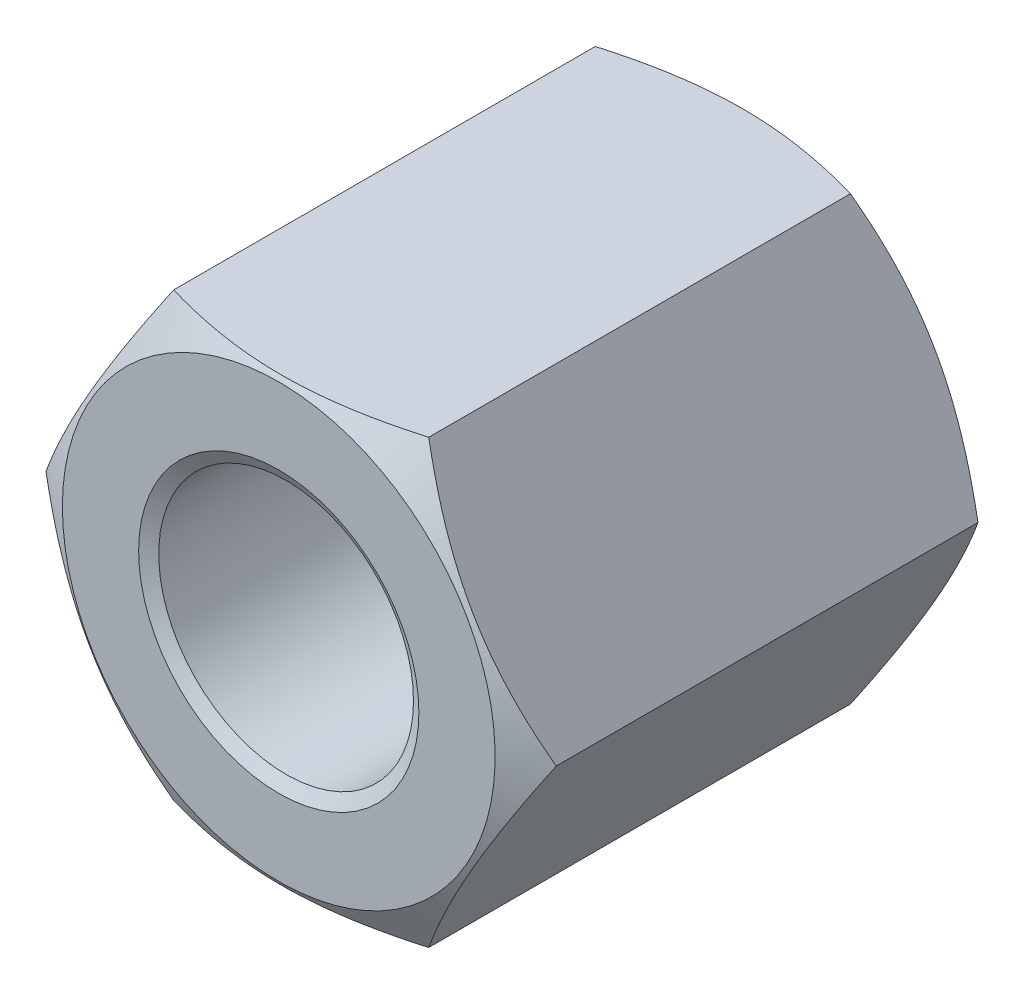
from build123d import *
from OCP.BRepFilletAPI import BRepFilletAPI_MakeChamfer

# Parameters (mm, degrees)
SKETCH1_R        = 10.376
BASENUT_DEPTH    = 38
ENDCHAMFER_SIZE  = 1.0376
ENDCHAMFER_SIZE2 = 0.599058639


with BuildPart() as part:
    # Sketch1 → BaseNut (new body)
    with BuildSketch(Plane.XY):
        Polygon((10.392304845, -18), (20.784609691, 0), (10.392304845, 18), (-10.392304845, 18), (-20.784609691, 0), (-10.392304845, -18), align=None)
        Circle(SKETCH1_R, mode=Mode.SUBTRACT)
    extrude(amount=-BASENUT_DEPTH)

    # Sketch2 → Double-Chamfer (revolve, cut)
    with BuildSketch(Plane(origin=(0, 0, 0), x_dir=(1, 0, 0), z_dir=(0, 1, 0))):
        Polygon((-20.784609691, 38), (-17.625, 38), (-20.784609691, 36.175798494), align=None)
        Polygon((-20.784609691, 1.824201506), (-20.784609691, 0), (-17.625, 0), align=None)
    revolve(axis=Axis((0, 0, -3.375940562), (0, 0, 1)), mode=Mode.SUBTRACT)

    # EndChamfer: one chamfer whose edges measure the first distance from different faces: ONE call of the kernel's chamfer builder (chamfer() names one face for all edges)
    endchamfer_edges_1 = [part.edges().sort_by_distance(p)[0] for p in [
        (-10.376, 0, -38),
    ]]
    endchamfer_side_1 = [part.faces().sort_by_distance(p)[0] for p in [
        (-10.376, 0, -19),
    ]]
    endchamfer_edges_2 = [part.edges().sort_by_distance(p)[0] for p in [
        (-10.376, 0, 0),
    ]]
    endchamfer_side_2 = [part.faces().sort_by_distance(p)[0] for p in [
        (17.126489719, 0, 0),
    ]]
    endchamfer = BRepFilletAPI_MakeChamfer(part.part.solid().wrapped)
    for e in endchamfer_edges_1:
        endchamfer.Add(ENDCHAMFER_SIZE, ENDCHAMFER_SIZE2, e.wrapped, endchamfer_side_1[0].wrapped)  # the first distance lies on this face
    for e in endchamfer_edges_2:
        endchamfer.Add(ENDCHAMFER_SIZE, ENDCHAMFER_SIZE2, e.wrapped, endchamfer_side_2[0].wrapped)  # the first distance lies on this face
    add(Compound.cast(endchamfer.Shape()), mode=Mode.REPLACE)


solid = part.part
